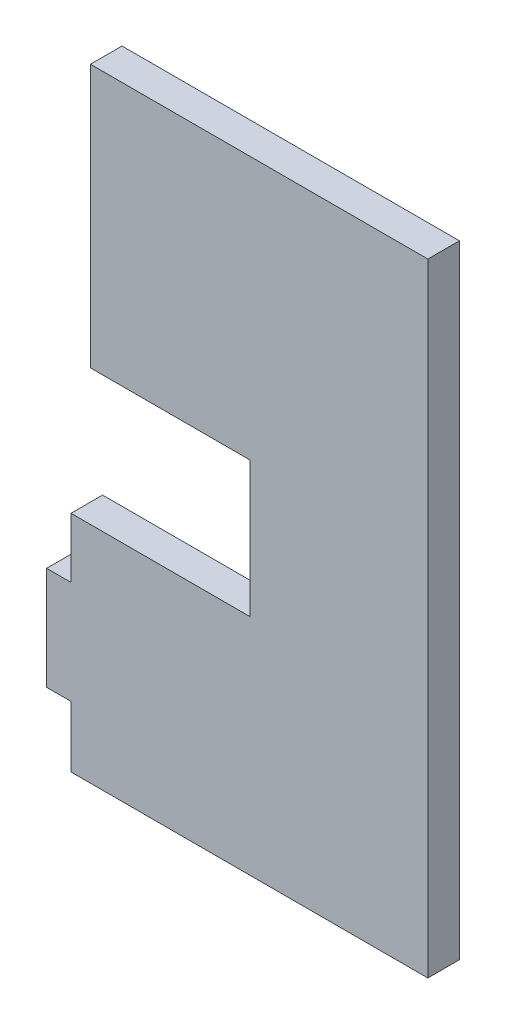
from build123d import *

# Parameters (mm, degrees)
BOSS_EXTRUDE1_DEPTH = 3


with BuildPart() as part:
    # Sketch1 → Boss-Extrude1 (new body)
    with BuildSketch(Plane.XY):
        Polygon((3, -18.58433147), (0.680763745, -18.58433147), (0.680763745, -28.385118219), (3, -28.385118219), (3, -34.192991848), (36.923110286, -34.192991848), (36.923110286, 25), (4.847061595, 25), (4.847061595, 0), (20, 0), (20, -12.894618578), (3, -12.894618578), align=None)
    extrude(amount=BOSS_EXTRUDE1_DEPTH)


solid = part.part
